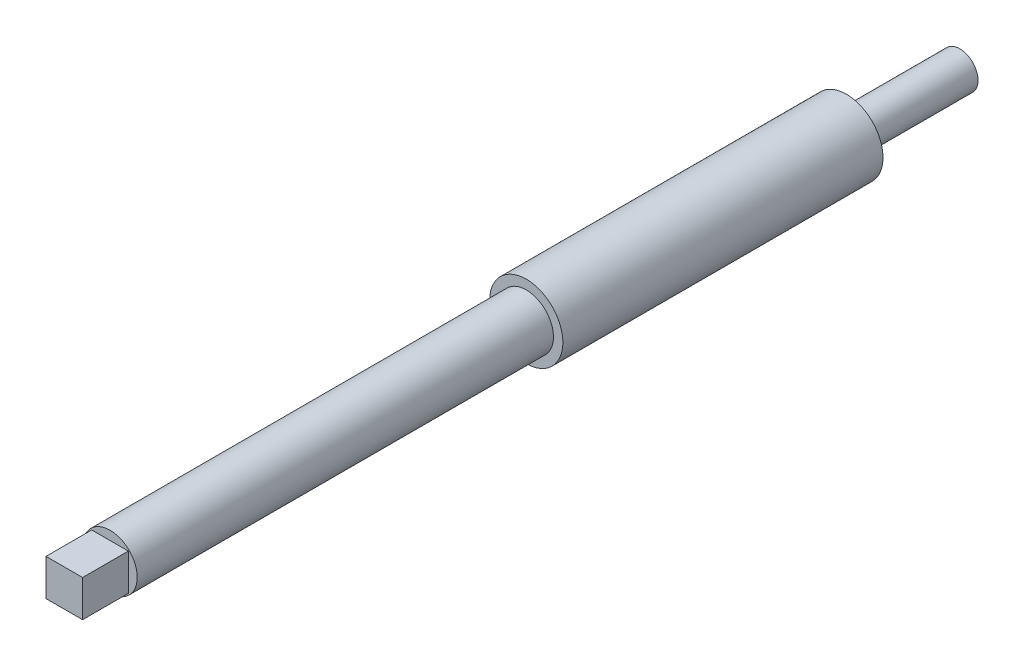
SolidWorks part; units mm, degrees
ref_plane "前视基准面" through (0, 0, 0) normal (0, 0, 1) x (1, 0, 0)
ref_plane "上视基准面" through (0, 0, 0) normal (0, 1, 0) x (1, 0, 0)
ref_plane "右视基准面" through (0, 0, 0) normal (1, 0, 0) x (0, 0, -1)
sketch "草图1" plane through (0, 0, 0) normal (0, 0, 1) x (1, 0, 0)
  circle A0 centre (0, 0) radius 5.95
  dimension "D1" = 11.9
extrude "凸台-拉伸1" add sketch "草图1" along normal blind 91
sketch "草图2" plane through (0, 0, 91) normal (0, 0, 1) x (1, 0, 0)
  line L1 (4, 4) -> (-4, 4)
  line L2 (4, 4) -> (4, -4)
  line L3 (4, -4) -> (-4, -4)
  line L4 (-4, 4) -> (-4, -4)
  line L5 (4, 4) -> (-4, -4) construction
  line L6 (4, -4) -> (-4, 4) construction
  point P0 (0, 0)
  dimension "D1" = 8
  dimension "D2" = 8
extrude "凸台-拉伸2" add sketch "草图2" along normal blind 10
sketch "草图3" plane through (0, 0, 0) normal (0, 0, -1) x (-1, 0, 0)
  circle A0 centre (0, 0) radius 8
extrude "凸台-拉伸3" add sketch "草图3" along normal blind 70
sketch "草图4" plane through (0, 0, -70) normal (0, 0, -1) x (-1, 0, 0)
  circle A0 centre (0.2246, 0) radius 4
  dimension "D1" = 8
extrude "凸台-拉伸4" add sketch "草图4" along normal blind 25
cosmetic thread "装饰螺纹线1" parameters "D2"=7
